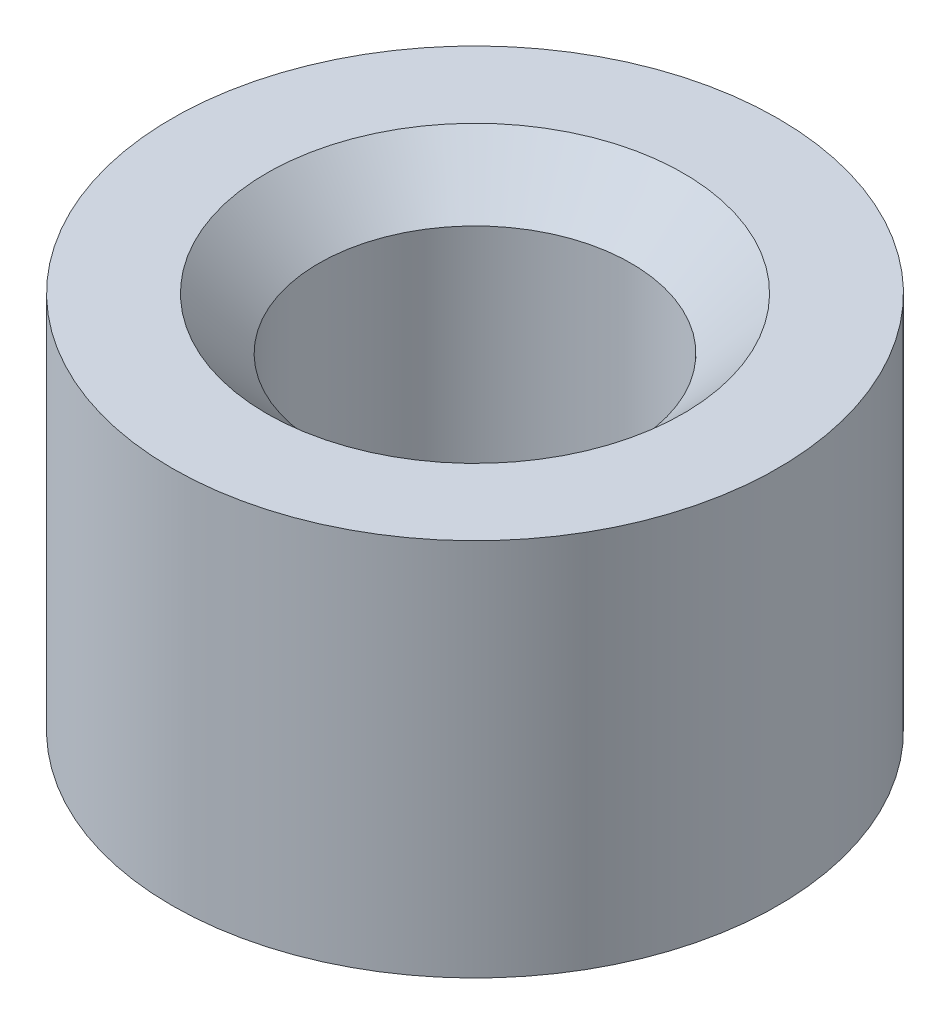
SolidWorks part; units mm, degrees
material "Q235"
ref_plane "Front Plane" through (0, 0, 0) normal (0, 0, 1) x (1, 0, 0)
ref_plane "Top Plane" through (0, 0, 0) normal (0, 1, 0) x (1, 0, 0)
ref_plane "Right Plane" through (0, 0, 0) normal (1, 0, 0) x (0, 0, -1)
sketch "Sketch1" plane through (0, 0, 0) normal (0, 1, 0) x (1, 0, 0)
  circle A0 centre (0, 0) radius 16
  circle A1 centre (0, 0) radius 7.5
  dimension "D1" = 32
  dimension "D2" = 15
extrude "Boss-Extrude1" add sketch "Sketch1" along normal blind 20
hole_wizard "M18x1.5 Tapped Hole2" positions "Sketch4" profile "Sketch5" tap size "M18x1.5" standard "GB"
sketch "Sketch4" plane through (0, 20, 0) normal (0, 1, 0) x (1, 0, 0)
  point P0 (0, 0)
sketch "Sketch5" plane through (0, 20, 0) normal (1, 0, 0) x (0, 0, 1)
  line L0 (0, 0) -> (0, 34.9571)
  line L1 (0, 34.9571) -> (8.25, 30)
  line L2 (8.25, 30) -> (8.25, 0)
  line L5 (8.25, 0) -> (0, 0)
  line L10 (0, 34.9571) -> (-8.25, 30) construction
  line L11 (0, -6.35) -> (0, 107.95) construction
  dimension "螺纹孔钻头直径" = 16.5
  dimension "螺纹孔钻头深度" = 30
  dimension "导头角度" = 118
cosmetic thread "Hole cosmetic thread2" parameters "D1"=20, "D2"=18
chamfer "Chamfer1" distance 2.75 angle 45 1 edges at (0, 20, 8.25)
